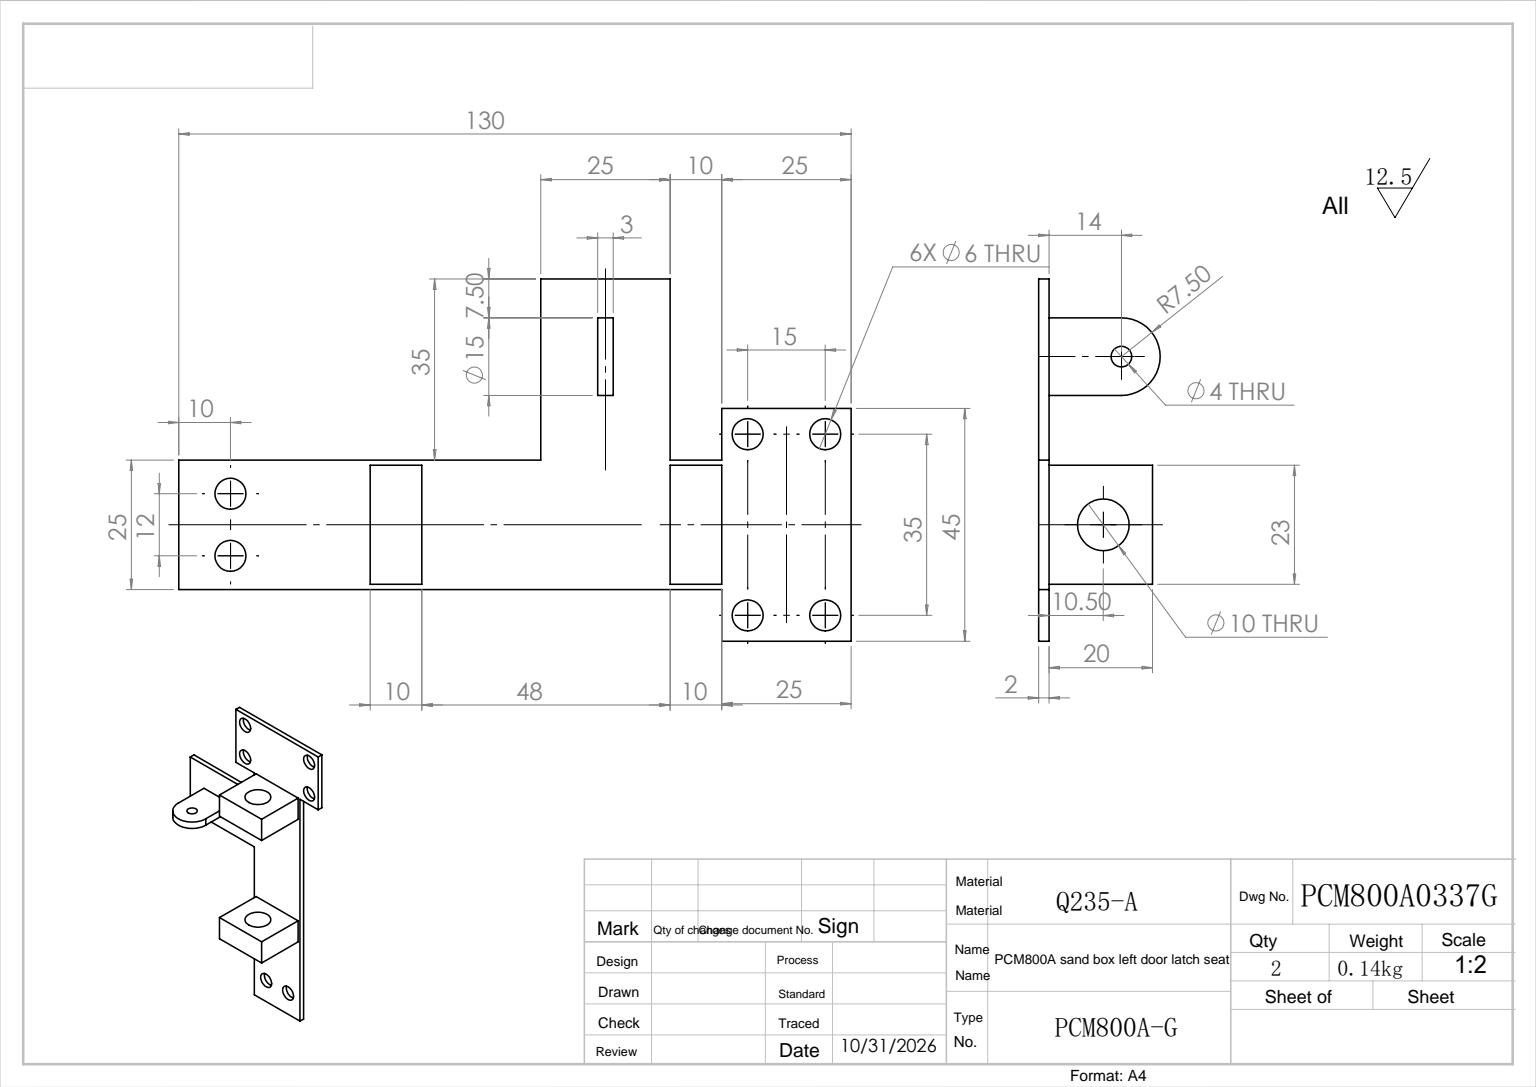
SolidWorks part; units mm, degrees
ref_plane "前视基准面" through (0, 0, 0) normal (0, 0, 1) x (1, 0, 0)
ref_plane "上视基准面" through (0, 0, 0) normal (0, 1, 0) x (1, 0, 0)
ref_plane "右视基准面" through (0, 0, 0) normal (1, 0, 0) x (0, 0, -1)
sketch "草图1" plane through (0, 0, 0) normal (0, 0, 1) x (1, 0, 0)
  line L0 (0, 0) -> (45, 0)
  line L1 (45, 0) -> (45, -25)
  line L2 (45, -25) -> (35, -25)
  line L3 (35, -25) -> (35, -130)
  line L4 (35, -130) -> (10, -130)
  line L5 (10, -130) -> (10, -60)
  line L6 (10, -60) -> (-25, -60)
  line L7 (-25, -60) -> (-25, -35)
  line L8 (-25, -35) -> (10, -35)
  line L9 (10, -35) -> (10, -25)
  line L10 (10, -25) -> (0, -25)
  line L11 (0, -25) -> (0, 0)
  circle A0 centre (5, -5) radius 3
  circle A1 centre (40, -5) radius 3
  circle A2 centre (5, -20) radius 3
  circle A3 centre (40, -20) radius 3
  circle A4 centre (16.5, -120) radius 3
  circle A5 centre (28.5, -120) radius 3
  dimension "D8" = 6
  dimension "D11" = 5
  dimension "D12" = 5
  dimension "D13" = 6
  dimension "D14" = 10
  dimension "D15" = 6.5
  dimension "D1" = 45
  dimension "D2" = 10
  dimension "D3" = 10
  dimension "D4" = 25
  dimension "D5" = 25
  dimension "D6" = 35
  dimension "D7" = 130
  dimension "D17" = 10
  dimension "D9" = 2
  dimension "D10" = 2
  dimension "D16" = 2
extrude "凸台-拉伸1" add sketch "草图1" along normal blind 2
sketch "草图2" plane through (0, 0, 0) normal (0, 1, 0) x (1, 0, 0)
  line L0 (45, -2) -> (0, -2) construction
  line L1 (11, -2) -> (34, -2)
  line L2 (11, -2) -> (11, -22)
  line L3 (11, -22) -> (34, -22)
  line L4 (34, -2) -> (34, -22)
  line L5 (45, -2) -> (45, 0) construction
  circle A0 centre (22.5, -12.5) radius 5
  dimension "D4" = 10
  dimension "D5" = 10.5
  dimension "D1" = 23
  dimension "D2" = 20
  dimension "D3" = 11
extrude "凸台-拉伸2" add sketch "草图2" against normal blind 10 from offset 25 offset against normal yes
pattern_linear "阵列(线性)1" count 2 spacing 58 along (0, -1, 0) of "凸台-拉伸2"
sketch "草图3" plane through (0, -35, 0) normal (0, 1, 0) x (1, 0, 0)
  line L0 (10, -2) -> (-25, -2) construction
  line L1 (-17.5, -2) -> (-2.5, -2)
  line L2 (-17.5, -2) -> (-17.5, -16)
  line L4 (-2.5, -2) -> (-2.5, -16)
  line L5 (-25, -2) -> (-25, 0) construction
  arc A0 (-17.5, -16) -> (-2.5, -16) centre (-10, -16) ccw
  circle A1 centre (-10, -16) radius 2
  dimension "D3" = 15
  dimension "D4" = 7.5
  dimension "D5" = 4
  dimension "D1" = 15
  dimension "D2" = 14
extrude "凸台-拉伸3" add sketch "草图3" against normal blind 3 from offset 11 offset against normal yes
